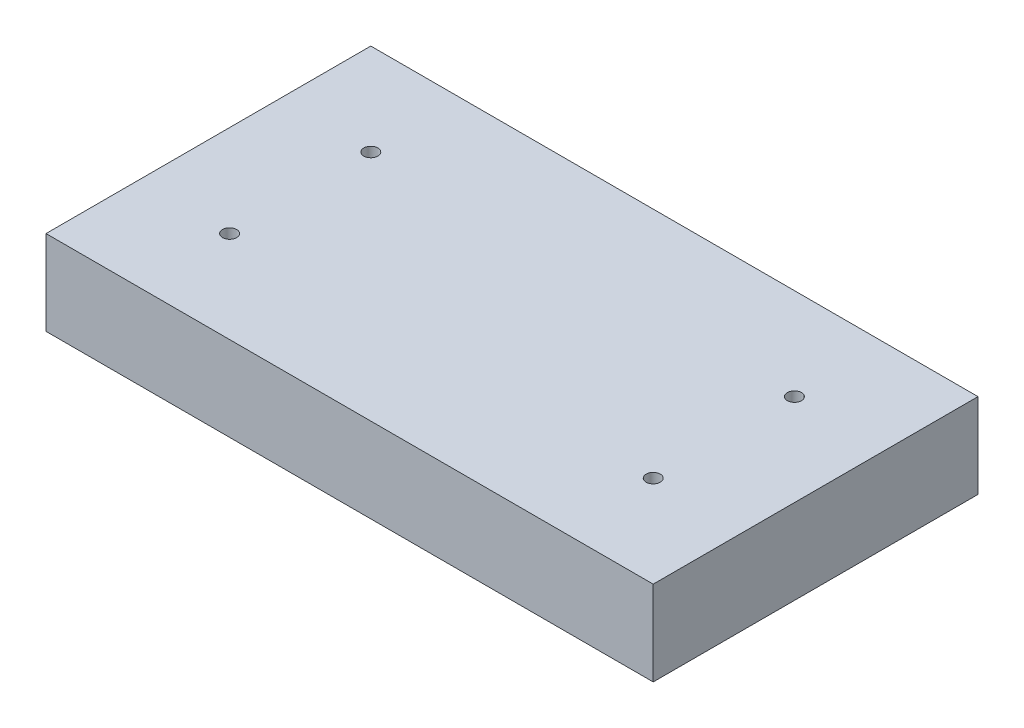
SolidWorks part; units mm, degrees
ref_plane "前视基准面" through (0, 0, 0) normal (0, 0, 1) x (1, 0, 0)
ref_plane "上视基准面" through (0, 0, 0) normal (0, 1, 0) x (1, 0, 0)
ref_plane "右视基准面" through (0, 0, 0) normal (1, 0, 0) x (0, 0, -1)
sketch "草图1" plane through (0, 0, 0) normal (0, 1, 0) x (1, 0, 0)
  line L1 (-107.5, 57.5) -> (107.5, 57.5)
  line L2 (-107.5, 57.5) -> (-107.5, -57.5)
  line L3 (-107.5, -57.5) -> (107.5, -57.5)
  line L4 (107.5, 57.5) -> (107.5, -57.5)
  line L5 (-107.5, 57.5) -> (107.5, -57.5) construction
  line L6 (-107.5, -57.5) -> (107.5, 57.5) construction
  point P0 (0, 0)
  dimension "D1" = 115
  dimension "D2" = 215
extrude "凸台-拉伸1" add sketch "草图1" along normal blind 30
sketch "草图2" plane through (0, 30, 0) normal (0, 1, 0) x (1, 0, 0)
  line L1 (-75, 25) -> (75, 25) construction
  line L2 (-75, 25) -> (-75, -25) construction
  line L3 (-75, -25) -> (75, -25) construction
  line L4 (75, 25) -> (75, -25) construction
  line L5 (-75, 25) -> (75, -25) construction
  line L6 (-75, -25) -> (75, 25) construction
  circle A0 centre (-75, 25) radius 2.5
  circle A1 centre (75, 25) radius 2.5
  circle A2 centre (75, -25) radius 2.5
  circle A3 centre (-75, -25) radius 2.5
  point P0 (0, 0)
  dimension "D1" = 5
  dimension "D2" = 50
  dimension "D3" = 150
extrude "切除-拉伸1" cut sketch "草图2" against normal blind 30
